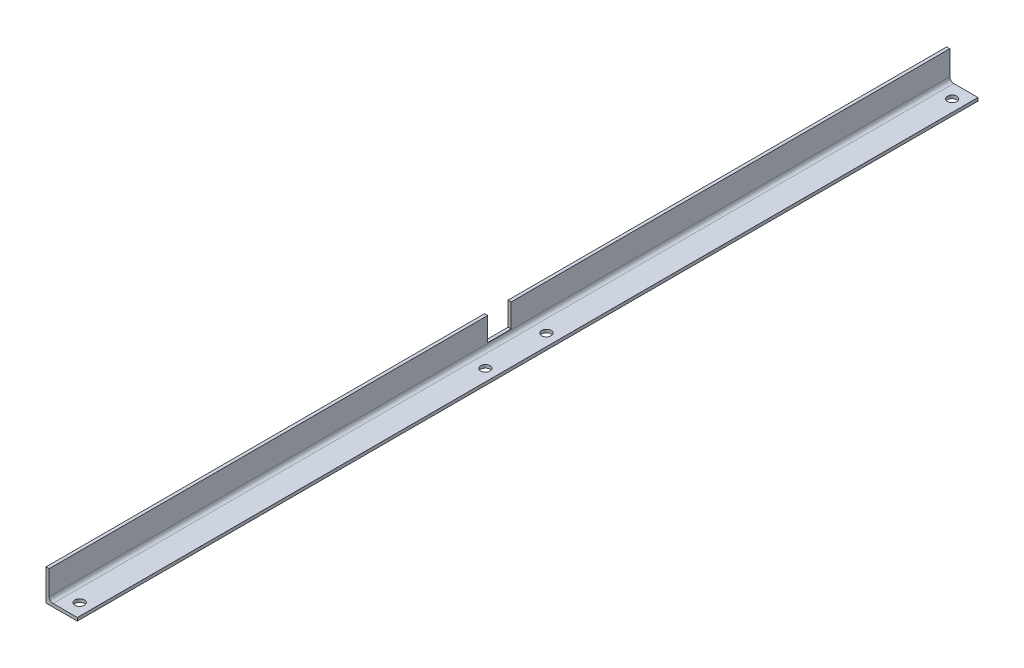
from build123d import *

# Parameters (mm, degrees)
EXTRUDE_1_DEPTH         = 1150
HOLE_WIZARD_12_0_12_1_D = 12
SKETCH_4_W              = 30
SKETCH_4_H              = 50.480703337
CUT_EXTRUDE_1_DEPTH     = 10


with BuildPart() as part:
    # 草图1 → 拉伸1 (new body)
    with BuildSketch(Plane.XY):
        with BuildLine():
            Line((0, 0), (0, 40))
            Line((0, 40), (3.99, 40))
            ThreePointArc((3.99, 40), (3.997071068, 39.997071068), (4, 39.99))
            Line((4, 39.99), (4, 9))
            ThreePointArc((4, 9), (5.464466094, 5.464466094), (9, 4))
            Line((9, 4), (39.99, 4))
            ThreePointArc((39.99, 4), (39.997071068, 3.997071068), (40, 3.99))
            Line((40, 3.99), (40, 0))
            Line((40, 0), (0, 0))
        make_face()
    extrude(amount=EXTRUDE_1_DEPTH)

    # Ø12.0 (12) 直径孔1 (through all)
    with Locations(Plane(origin=(0, 4, 0), x_dir=(1, 0, 0), z_dir=(0, 1, 0))):
        with Locations((24.99, -1132), (24.99, -614), (24.99, -536), (24.99, -18)):
            Hole(HOLE_WIZARD_12_0_12_1_D / 2)

    # 草图4 → 切除-拉伸1 (cut)
    with BuildSketch(Plane(origin=(4, 0, 0), x_dir=(0, 0, -1), z_dir=(1, 0, 0))):
        with Locations((-575, 35.240351668)):
            Rectangle(SKETCH_4_W, SKETCH_4_H)
    extrude(amount=-CUT_EXTRUDE_1_DEPTH, mode=Mode.SUBTRACT)


solid = part.part
